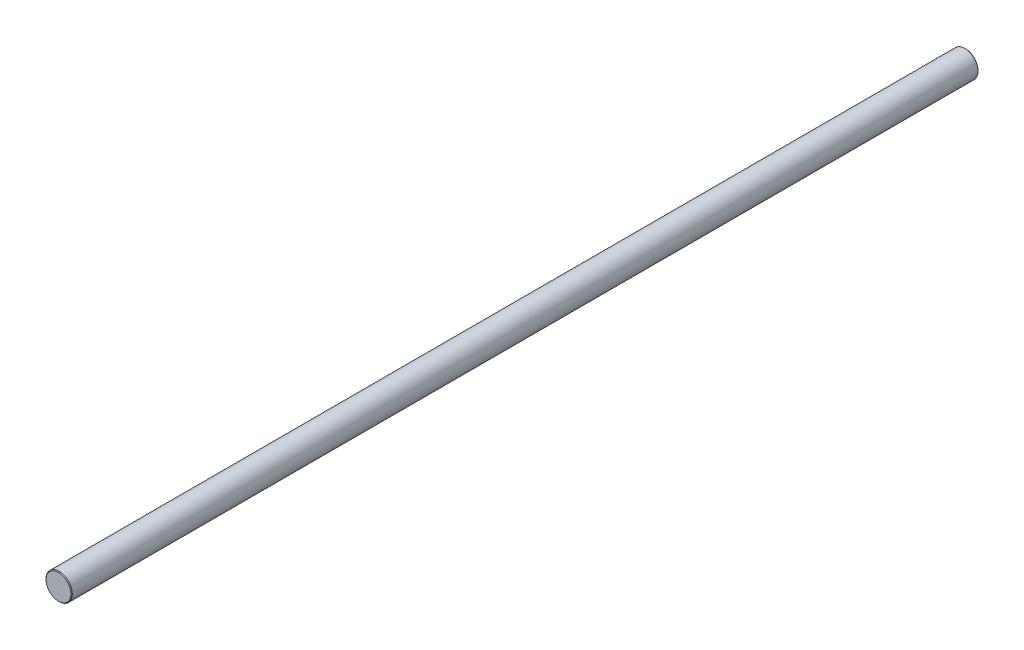
SolidWorks part; units mm, degrees
material "Q235A"
ref_plane "前基準面" through (0, 0, 0) normal (0, 0, 1) x (1, 0, 0)
ref_plane "上基準面" through (0, 0, 0) normal (0, 1, 0) x (1, 0, 0)
ref_plane "右基準面" through (0, 0, 0) normal (1, 0, 0) x (0, 0, -1)
sketch "草图1" plane through (0, 0, 0) normal (0, 0, 1) x (1, 0, 0)
  circle A0 centre (0, 0) radius 10
  dimension "D1" = 20
extrude "凸台-拉伸1" add sketch "草图1" along normal mid plane 690
chamfer "倒角1" distance 0.5 angle 45 2 edges at (10, 0, -345) (10, 0, 345)
